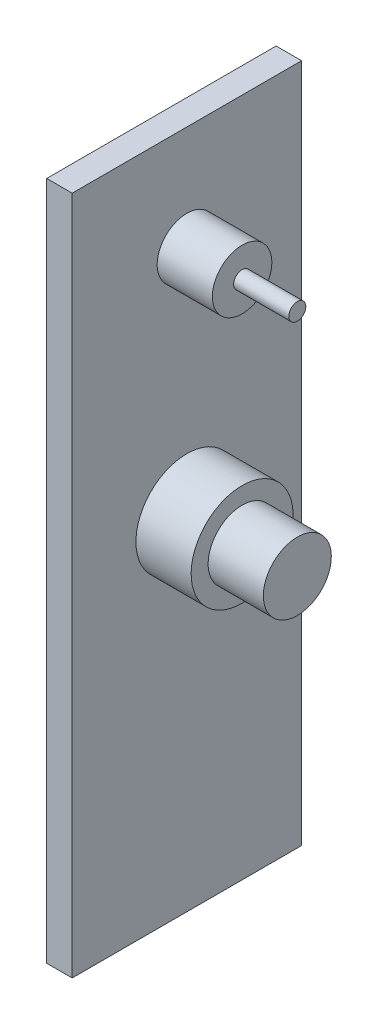
SolidWorks part; units mm, degrees
ref_plane "前视基准面" through (0, 0, 0) normal (0, 0, 1) x (1, 0, 0)
ref_plane "上视基准面" through (0, 0, 0) normal (0, 1, 0) x (1, 0, 0)
ref_plane "右视基准面" through (0, 0, 0) normal (1, 0, 0) x (0, 0, -1)
sketch "草图1" plane through (0, 0, 0) normal (0, 0, 1) x (1, 0, 0)
  line L1 (-0.9828, 79.0713) -> (2.0172, 79.0713)
  line L2 (-0.9828, 79.0713) -> (-0.9828, -0.9287)
  line L3 (-0.9828, -0.9287) -> (2.0172, -0.9287)
  line L4 (2.0172, 79.0713) -> (2.0172, -0.9287)
  dimension "D1" = 3
  dimension "D2" = 80
extrude "凸台-拉伸1" add sketch "草图1" along normal blind 27
sketch "草图2" plane through (2.0172, 0, 0) normal (1, 0, 0) x (0, 0, -1)
  line L0 (-27, -0.9287) -> (0, -0.9287) construction
  circle A0 centre (-13.5, 66.7713) radius 3.5
  circle A1 centre (-13.5, 39.7713) radius 6
  dimension "D1" = 12
  dimension "D3" = 7
  dimension "D2" = 40.7
  dimension "D4" = 67.7
extrude "凸台-拉伸2" add sketch "草图2" along normal blind 6.5
sketch "草图3" plane through (8.5172, 0, 0) normal (1, 0, 0) x (0, 0, -1)
  circle A0 centre (-13.5, 66.7713) radius 1
  circle A1 centre (-13.5, 39.7713) radius 4
  dimension "D1" = 2
  dimension "D2" = 8
extrude "凸台-拉伸3" add sketch "草图3" along normal blind 6.5
extrude "切除-拉伸1" cut sketch "草图4" against normal blind 15
sketch "草图4" plane through (-1096.2139, -10.9287, 855.0606) normal (0, -1, 0) x (0.1219, 0, -0.9925)
  line L0 (957.1306, 1000.5442) -> (983.9293, 997.2537) construction
  line L3 (955.5463, 987.6411) -> (982.345, 984.3506) construction
  circle A0 centre (963.0859, 999.813) radius 1
  circle A1 centre (977.9741, 997.9849) radius 1
  circle A2 centre (961.5016, 986.9099) radius 1
  circle A3 centre (976.3898, 985.0818) radius 1
sketch "草图5" plane through (0, -0.9287, 0) normal (0, -1, 0) x (1, 0, 0)
  circle A0 centre (0.5172, 21) radius 1
  circle A1 centre (0.5172, 6) radius 1
